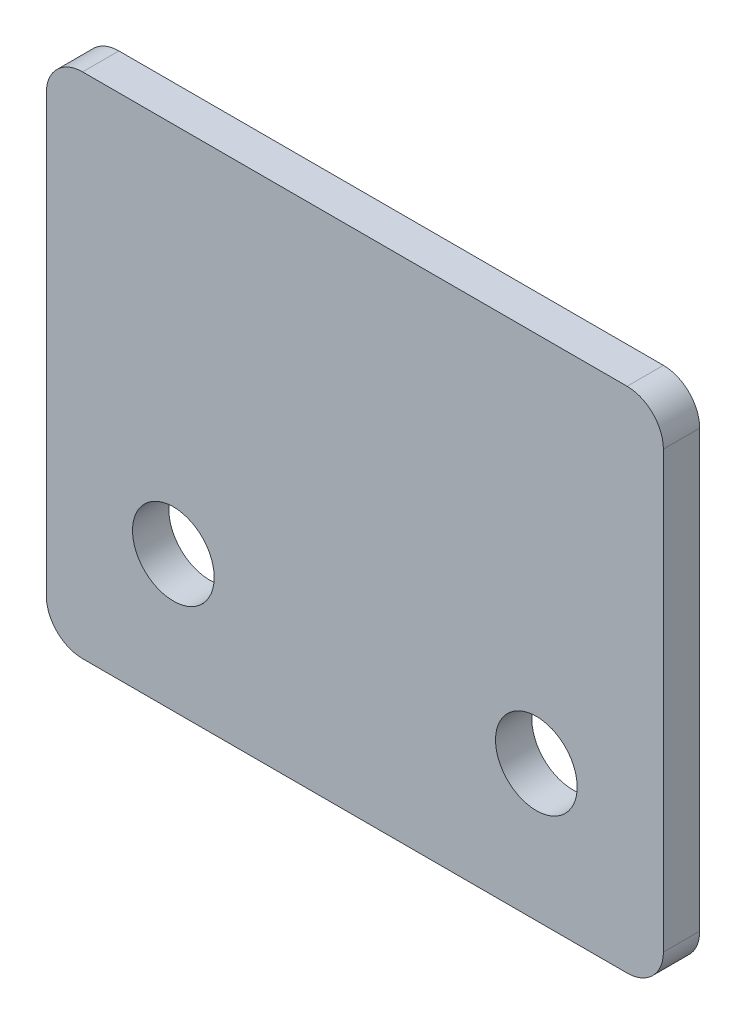
from build123d import *

# Parameters (mm, degrees)
SKETCH1_W           = 34
SKETCH1_H           = 28
SKETCH1_R           = 2.25
BOSS_EXTRUDE1_DEPTH = 2
FILLET1_R           = 2


with BuildPart() as part:
    # Sketch1 → Boss-Extrude1 (new body)
    with BuildSketch(Plane.XY):
        with Locations((0, 14)):
            Rectangle(SKETCH1_W, SKETCH1_H)
        with Locations((-10, 7.5)):
            Circle(SKETCH1_R, mode=Mode.SUBTRACT)
        with Locations(Location((10, 7.5, 0), (0, 0, 180))):
            Circle(SKETCH1_R, mode=Mode.SUBTRACT)
    extrude(amount=BOSS_EXTRUDE1_DEPTH)

    # Fillet1
    fillet1_edges = [part.edges().sort_by_distance(p)[0] for p in [
        (17, 0, 1),
        (-17, 0, 1),
        (-17, 28, 1),
        (17, 28, 1),
    ]]
    fillet(fillet1_edges, radius=FILLET1_R)


solid = part.part
